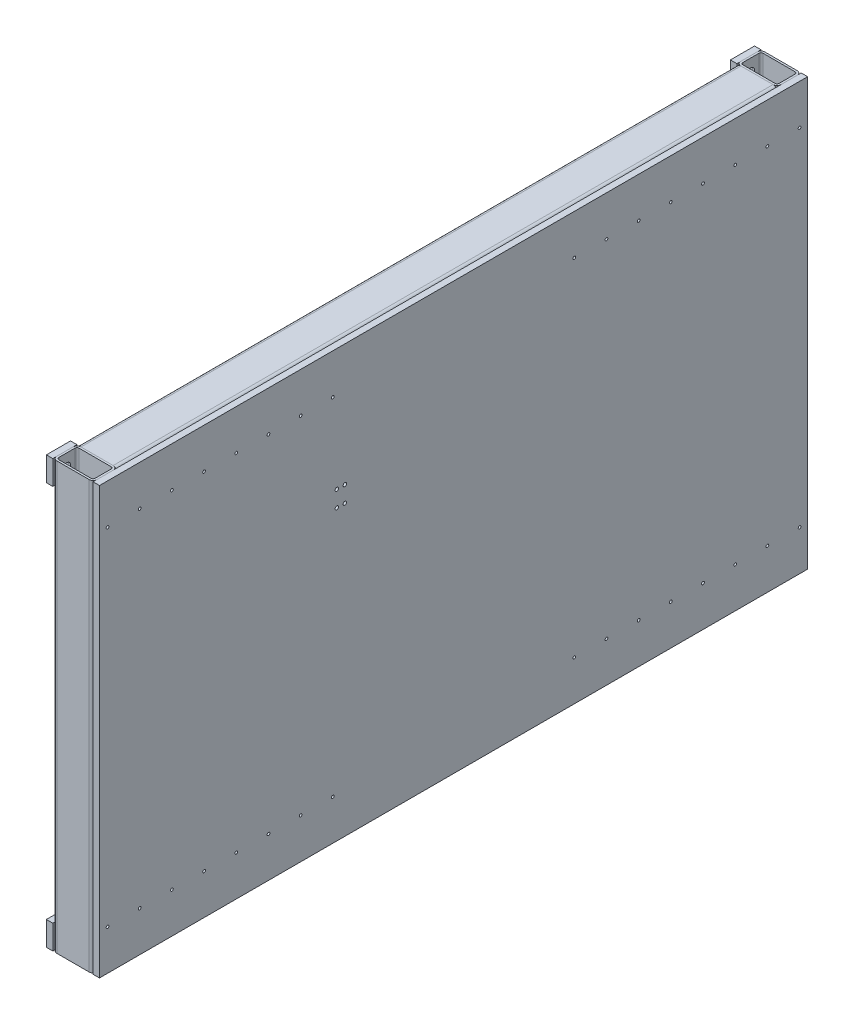
SolidWorks part; units mm, degrees
ref_plane "前视基准面" through (0, 0, 0) normal (0, 0, 1) x (1, 0, 0)
ref_plane "上视基准面" through (0, 0, 0) normal (0, 1, 0) x (1, 0, 0)
ref_plane "右视基准面" through (0, 0, 0) normal (1, 0, 0) x (0, 0, -1)
sketch "草图2" plane through (0, 0, 0) normal (1, 0, 0) x (0, 0, -1)
  line L0 (-850, 200) -> (850, 200)
  line L1 (-850, 500) -> (850, 500)
  line L2 (-850, 500) -> (-850, -500)
  line L3 (-850, -500) -> (850, -500)
  line L4 (850, 500) -> (850, -500)
  line L5 (-850, 500) -> (850, -500) construction
  line L6 (-850, -500) -> (850, 500) construction
  line L7 (-850, -200) -> (850, -200)
  line L8 (-850, 0) -> (743.9235, 0) construction
  point P0 (0, 0)
  dimension "D1" = 1700
  dimension "D2" = 1000
  dimension "D3" = 400
other "矩型管 100 X 60 X 5.0(1)"
ref_plane "基准面1" through (0, 500, 850) normal (0, -1, 0) x (0, 0, -1)
sketch "Sketch1" plane through (0, 500, 850) normal (0, -1, 0) x (0, 0, -1)
  line L0 (-20, -45) -> (20, -45)
  line L1 (-25, -40) -> (-25, 40)
  line L2 (20, 45) -> (-20, 45)
  line L3 (25, 40) -> (25, -40)
  line L4 (-20, -50) -> (20, -50)
  line L5 (-30, -40) -> (-30, 40)
  line L6 (20, 50) -> (-20, 50)
  line L7 (30, 40) -> (30, -40)
  line L8 (-30, 0) -> (-25, 0) construction
  line L9 (-25, 0) -> (25, 0) construction
  line L10 (25, 0) -> (30, 0) construction
  line L11 (0, 50) -> (0, 45) construction
  line L12 (0, 45) -> (0, -45) construction
  line L13 (0, -45) -> (0, -50) construction
  arc A0 (30, 40) -> (20, 50) centre (20, 40) ccw
  arc A1 (20, -50) -> (30, -40) centre (20, -40) ccw
  arc A2 (-30, -40) -> (-20, -50) centre (-20, -40) ccw
  arc A3 (-20, 50) -> (-30, 40) centre (-20, 40) ccw
  arc A4 (-20, 45) -> (-25, 40) centre (-20, 40) ccw
  arc A5 (25, 40) -> (20, 45) centre (20, 40) ccw
  arc A6 (20, -45) -> (25, -40) centre (20, -40) ccw
  arc A7 (-25, -40) -> (-20, -45) centre (-20, -40) ccw
  point P6 (-30, 50)
  point P33 (-30, -50)
  point P34 (30, -50)
  point P36 (30, 50)
  point P37 (0, 0)
  dimension "D1" = 10
  dimension "Thickness" = 5
  dimension "V_leg" = 100
  dimension "H_leg" = 60
sketch "草图4" plane through (50, 0, 0) normal (1, 0, 0) x (0, 0, -1)
  line L1 (-880, 530) -> (880, 530)
  line L2 (-880, 530) -> (-880, -530)
  line L3 (-880, -530) -> (880, -530)
  line L4 (880, 530) -> (880, -530)
extrude "凸台-拉伸1" add sketch "草图4" along normal blind 16 separate body
sketch "草图5" plane through (-50, 0, 0) normal (-1, 0, 0) x (0, 0, 1)
  line L0 (-820, 480) -> (-820, 470) construction
  line L1 (-880, 530) -> (-820, 530)
  line L2 (-880, 530) -> (-880, 470)
  line L3 (-880, 470) -> (-820, 470)
  line L4 (-820, 530) -> (-820, 470)
  line L5 (820, -530) -> (820, 530) construction
  line L6 (880, 530) -> (820, 530)
  line L7 (880, 530) -> (880, 470)
  line L8 (880, 470) -> (820, 470)
  line L9 (820, 530) -> (820, 470)
  line L10 (-820, 470) -> (820, 470) construction
extrude "凸台-拉伸2" add sketch "草图5" along normal blind 16 separate body
mirror "镜向3" about plane through (0, 0, 0) normal (0, 1, 0) of "凸台-拉伸2"
hole_wizard "M20 螺纹孔1" positions "草图7" profile "草图8" tap size "M20" standard "ISO"
sketch "草图7" plane through (-66, 0, 0) normal (-1, 0, 0) x (0, 0, 1)
  point P0 (-850, -500)
sketch "草图8" plane through (-66, -500, -850) normal (0, 1, 0) x (0, 0, 1)
  line L0 (0, 0) -> (0, 52.7575)
  line L1 (0, 52.7575) -> (8.75, 47.5)
  line L2 (8.75, 47.5) -> (8.75, 0)
  line L5 (8.75, 0) -> (0, 0)
  line L10 (0, 52.7575) -> (-8.75, 47.5) construction
  line L11 (0, -6.35) -> (0, 107.95) construction
  dimension "螺纹孔钻头直径" = 17.5
  dimension "螺纹孔钻头深度" = 47.5
  dimension "导头角度" = 118
cosmetic thread "孔螺蚊线1" parameters "D1"=21, "D2"=20
mirror "镜向9" about plane through (0, 0, 0) normal (0, 1, 0) of "M20 螺纹孔1"
mirror "镜向11" about plane through (0, 0, 0) normal (0, 0, 1) of "M20 螺纹孔1", "镜向9"
hole_wizard "M8 螺纹孔1" positions "草图9" profile "草图10" tap size "M8" standard "ISO"
sketch "草图9" plane through (66, 0, 0) normal (1, 0, 0) x (0, 0, -1)
  line L0 (-880, 530) -> (-880, -530) construction
  line L1 (880, 530) -> (-880, 530) construction
  point P0 (-860, 430)
  dimension "D1" = 20
  dimension "D3" = 100
sketch "草图10" plane through (66, 430, 860) normal (0, 1, 0) x (0, 0, -1)
  line L0 (0, 0) -> (0, 21.7929)
  line L1 (0, 21.7929) -> (3.4, 19.75)
  line L2 (3.4, 19.75) -> (3.4, 0)
  line L5 (3.4, 0) -> (0, 0)
  line L10 (0, 21.7929) -> (-3.4, 19.75) construction
  line L11 (0, -6.35) -> (0, 107.95) construction
  dimension "螺纹孔钻头直径" = 6.8
  dimension "螺纹孔钻头深度" = 19.75
  dimension "导头角度" = 118
cosmetic thread "孔螺蚊线3" parameters "D1"=16, "D2"=8
pattern_linear "阵列(线性)1" count 8 spacing 80 along (0, 0, -1) of "M8 螺纹孔1"
mirror "镜向12" about plane through (0, 0, 0) normal (0, 1, 0) of "阵列(线性)1", "M8 螺纹孔1"
mirror "镜向13" about plane through (0, 0, 0) normal (0, 0, 1) of "镜向12", "M8 螺纹孔1", "阵列(线性)1"
hole_wizard "M10 螺纹孔1" positions "草图11" profile "草图12" tap size "M10" standard "GB"
sketch "草图11" plane through (66, 0, 0) normal (1, 0, 0) x (0, 0, -1)
  line L0 (-880, 530) -> (-880, -530) construction
  line L1 (-880, -530) -> (880, -530) construction
  point P0 (-270.25, 227)
  point P2 (-270.25, 187)
  point P11 (-290.25, 227)
  point P13 (-290.25, 187)
  dimension "D1" = 40
  dimension "D2" = 609.75
  dimension "D3" = 717
  dimension "D4" = 20
sketch "草图12" plane through (66, 227, 270.25) normal (0, 1, 0) x (0, 0, -1)
  line L0 (0, 0) -> (0, 42.5537)
  line L1 (0, 42.5537) -> (4.25, 40)
  line L2 (4.25, 40) -> (4.25, 0)
  line L5 (4.25, 0) -> (0, 0)
  line L10 (0, 42.5537) -> (-4.25, 40) construction
  line L11 (0, -6.35) -> (0, 107.95) construction
  dimension "螺纹孔钻头直径" = 8.5
  dimension "螺纹孔钻头深度" = 40
  dimension "导头角度" = 118
cosmetic thread "孔螺蚊线4" parameters "D1"=16, "D2"=10
cosmetic thread "孔螺蚊线5" parameters "D1"=16, "D2"=10
cosmetic thread "孔螺蚊线6" parameters "D1"=16, "D2"=10
cosmetic thread "孔螺蚊线7" parameters "D1"=16, "D2"=10
